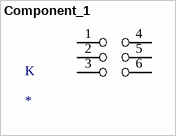
[diagram p0: symbol Component_1]
# Altium schematic symbol library MISC86340-30.SchLib: 1 symbol
Pins are listed as number, name and electrical type; pins without a type are passive.


## Component_1
designator K
footprint 自锁开关
pins: 1, 2, 3, 4, 5, 6